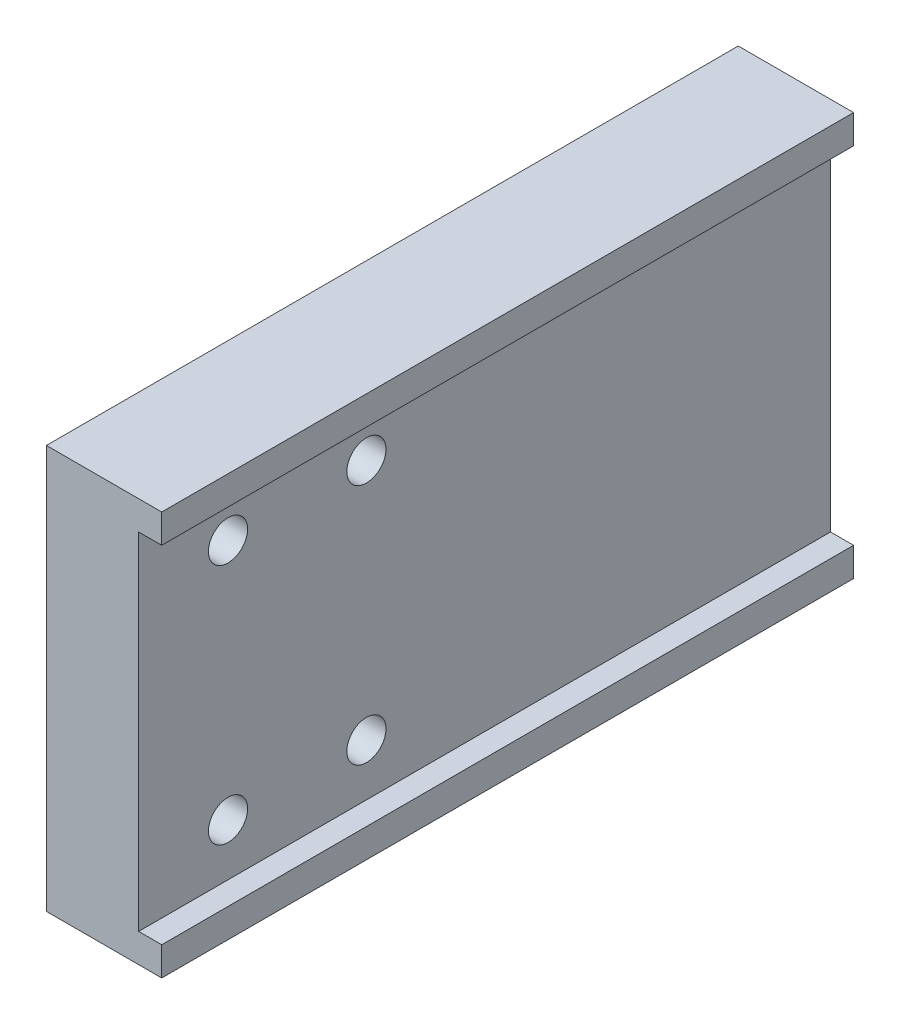
SolidWorks part; units mm, degrees
material "AL6061"
ref_plane "Front Plane" through (0, 0, 0) normal (0, 0, 1) x (1, 0, 0)
ref_plane "Top Plane" through (0, 0, 0) normal (0, 1, 0) x (1, 0, 0)
ref_plane "Right Plane" through (0, 0, 0) normal (1, 0, 0) x (0, 0, -1)
sketch "Sketch1" plane through (0, 0, 0) normal (1, 0, 0) x (0, 0, -1)
  line L1 (-30, -17.5) -> (30, -17.5)
  line L2 (-30, -17.5) -> (-30, 17.5)
  line L3 (-30, 17.5) -> (30, 17.5)
  line L4 (30, -17.5) -> (30, 17.5)
  line L5 (-30, -17.5) -> (30, 17.5) construction
  line L6 (-30, 17.5) -> (30, -17.5) construction
  point P0 (0, 0)
  dimension "D1" = 35
  dimension "D2" = 60
extrude "Boss-Extrude1" add sketch "Sketch1" along normal blind 10
sketch "Sketch2" plane through (10, 0, 0) normal (1, 0, 0) x (0, 0, -1)
  line L0 (30, 0) -> (-35.9, 0) construction
  line L1 (30, -17.5) -> (30, 17.5) construction
  line L2 (-35.9, 9) -> (-35.9, -9) construction
  line L3 (-30, 17.5) -> (-30, -17.5) construction
  line L4 (-30, 15) -> (30, 15)
  line L5 (-30, 15) -> (-30, -15)
  line L6 (-30, -15) -> (30, -15)
  line L7 (30, 15) -> (30, -15)
  line L8 (-30, 15) -> (30, -15) construction
  line L9 (-30, -15) -> (30, 15) construction
  point P6 (0, 0)
  dimension "D1" = 30
extrude "Cut-Extrude1" cut sketch "Sketch2" against normal blind 2
hole_wizard "CBORE for M3 Hexagon socket head cap screws1" positions "Sketch3" profile "Sketch4" counterbore size "M3" standard "GB" end condition through all
sketch "Sketch3" plane through (0, 0, 0) normal (-1, 0, 0) x (0, 0, 1)
  point P0 (22.25, 10.5)
  point P3 (10.25, 10.5)
  point P6 (10.25, -10.5)
  point P9 (22.25, -10.5)
sketch "Sketch4" plane through (0, 10.5, 22.25) normal (0, 1, 0) x (0, 0, 1)
  line L0 (0, 0) -> (0, 10)
  line L1 (0, 10) -> (1.7, 10)
  line L3 (1.7, 10) -> (1.7, 3.4)
  line L4 (1.7, 3.4) -> (3, 3.4)
  line L5 (3, 3.4) -> (3, 0)
  line L7 (3, 0) -> (0, 0)
  line L11 (0, -6.35) -> (0, 107.95) construction
  dimension "通孔孔直径" = 3.4
  dimension "通孔孔深度" = 10
  dimension "柱形沉头孔直径" = 6
  dimension "柱形沉头孔深度" = 3.4
hole_wizard "M4 Tapped Hole1" positions "Sketch5" profile "Sketch6" tap size "M4" standard "GB"
sketch "Sketch5" plane through (0, 0, -30) normal (0, 0, -1) x (-1, 0, 0)
  line L0 (-4, 17.5) -> (-4, -17.5) construction
  line L1 (-10, 17.5) -> (0, 17.5) construction
  line L2 (-10, -17.5) -> (0, -17.5) construction
  line L4 (0, -17.5) -> (0, 17.5) construction
  line L5 (0, 0) -> (-8, 0) construction
  line L6 (-8, -15) -> (-8, 15) construction
  point P18 (-4, 10)
  point P20 (-4, -10)
  dimension "D1" = 4
  dimension "D2" = 20
sketch "Sketch6" plane through (4, -10, -30) normal (1, 0, 0) x (0, 1, 0)
  line L0 (0, 0) -> (0, 11.0914)
  line L1 (0, 11.0914) -> (1.65, 10.1)
  line L2 (1.65, 10.1) -> (1.65, 0)
  line L5 (1.65, 0) -> (0, 0)
  line L10 (0, 11.0914) -> (-1.65, 10.1) construction
  line L11 (0, -6.35) -> (0, 107.95) construction
  dimension "螺纹孔钻头直径" = 3.3
  dimension "螺纹孔钻头深度" = 10.1
  dimension "导头角度" = 118
cosmetic thread "Cosmetic Thread1" parameters "D1"=8, "D2"=4
cosmetic thread "Cosmetic Thread2" parameters "D1"=8, "D2"=4
